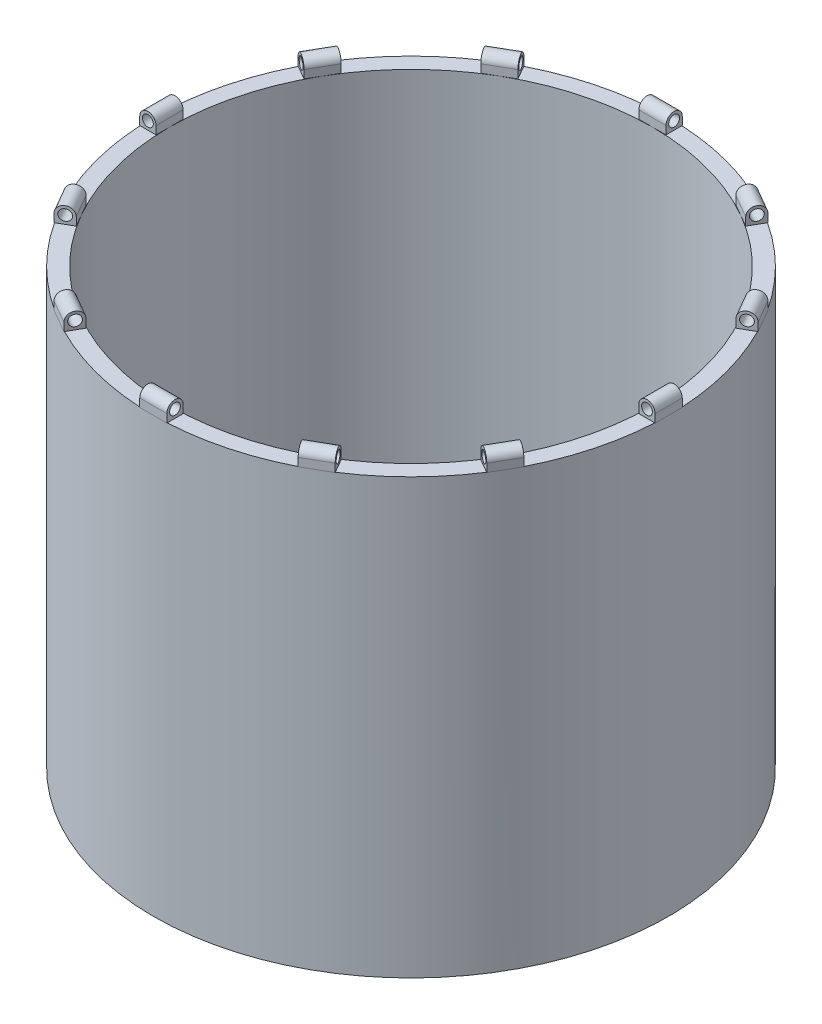
from build123d import *

# Parameters (mm, degrees)
SKETCH_1_R               = 47.5
SKETCH_1_R_2             = 44.5
EXTRUDE_1_DEPTH          = 80
SKETCH_2_R               = 1.5
SKETCH_2_R_2             = 1
EXTRUDE_3_DEPTH          = 2.5
PATTERN_CIRCULAR_1_COUNT = 12


with BuildPart() as part:
    # 草图1 → 凸台-拉伸1 (new body)
    with BuildSketch(Plane(origin=(0, 0, 0), x_dir=(1, 0, 0), z_dir=(0, 1, 0))):
        with Locations(Location((0, 0, 0), (0, 0, 270))):
            Circle(SKETCH_1_R)
        with Locations(Location((0, 0, 0), (0, 0, 270))):
            Circle(SKETCH_1_R_2, mode=Mode.SUBTRACT)
    extrude(amount=EXTRUDE_1_DEPTH)

    # 草图2 → 凸台-拉伸3 (add, symmetric)
    # profile 1 of 3: a face of its own
    with BuildSketch(Plane(origin=(0, 0, 0), x_dir=(0, 0, -1), z_dir=(1, 0, 0))):
        with BuildLine():
            ThreePointArc((-46, 80), (-47.060660172, 80.439339828), (-47.5, 81.5))
            Line((-47.5, 81.5), (-47.5, 80))
            Line((-47.5, 80), (-46, 80))
        make_face()
    # profile 2 of 3: a face of its own
    with BuildSketch(Plane(origin=(0, 0, 0), x_dir=(0, 0, -1), z_dir=(1, 0, 0))):
        with BuildLine():
            Line((-44.5, 80), (-44.5, 81.5))
            ThreePointArc((-44.5, 81.5), (-44.939339828, 80.439339828), (-46, 80))
            Line((-46, 80), (-44.5, 80))
        make_face()
    # profile 3 of 3: a face of its own
    with BuildSketch(Plane(origin=(0, 0, 0), x_dir=(0, 0, -1), z_dir=(1, 0, 0))):
        with Locations((-46, 81.5)):
            Circle(SKETCH_2_R)
        with Locations((-46, 81.5)):
            Circle(SKETCH_2_R_2, mode=Mode.SUBTRACT)
    extrude_3 = extrude(amount=EXTRUDE_3_DEPTH, both=True)

    # 阵列(圆周)1: 凸台-拉伸3 ×12 about axis
    pattern_circular_1_axis = Axis((0, 0, 0), (0, 1, 0))
    for i in range(1, PATTERN_CIRCULAR_1_COUNT):
        add(extrude_3.rotate(pattern_circular_1_axis, i * 360 / PATTERN_CIRCULAR_1_COUNT))


solid = part.part
